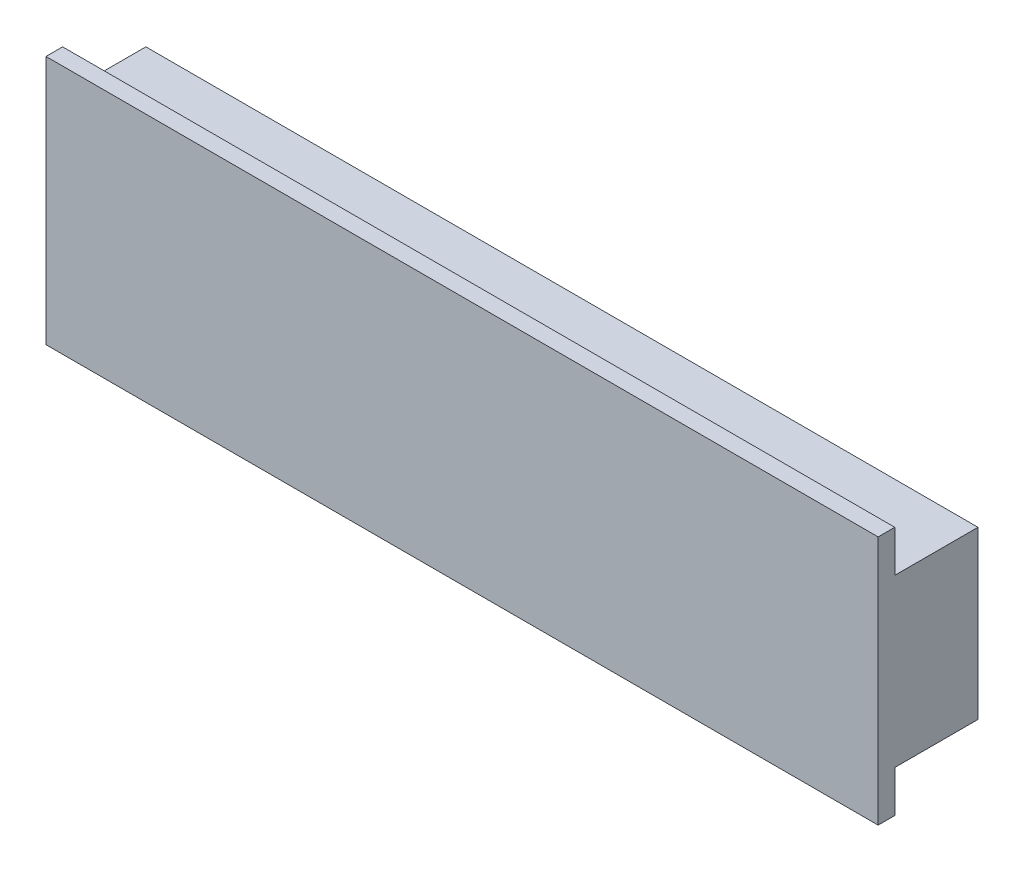
from build123d import *

# Parameters (mm, degrees)
SKETCH1_W           = 500
SKETCH1_H           = 150
BOSS_EXTRUDE1_DEPTH = 10
SKETCH2_W           = 500
SKETCH2_H           = 100
BOSS_EXTRUDE2_DEPTH = 50


with BuildPart() as part:
    # Sketch1 → Boss-Extrude1 (new body)
    with BuildSketch(Plane.XY):
        Rectangle(SKETCH1_W, SKETCH1_H)
    extrude(amount=BOSS_EXTRUDE1_DEPTH)

    # Sketch2 → Boss-Extrude2 (add)
    with BuildSketch(Plane(origin=(0, 0, 0), x_dir=(-1, 0, 0), z_dir=(0, 0, -1))):
        Rectangle(SKETCH2_W, SKETCH2_H)
    extrude(amount=BOSS_EXTRUDE2_DEPTH)


solid = part.part
